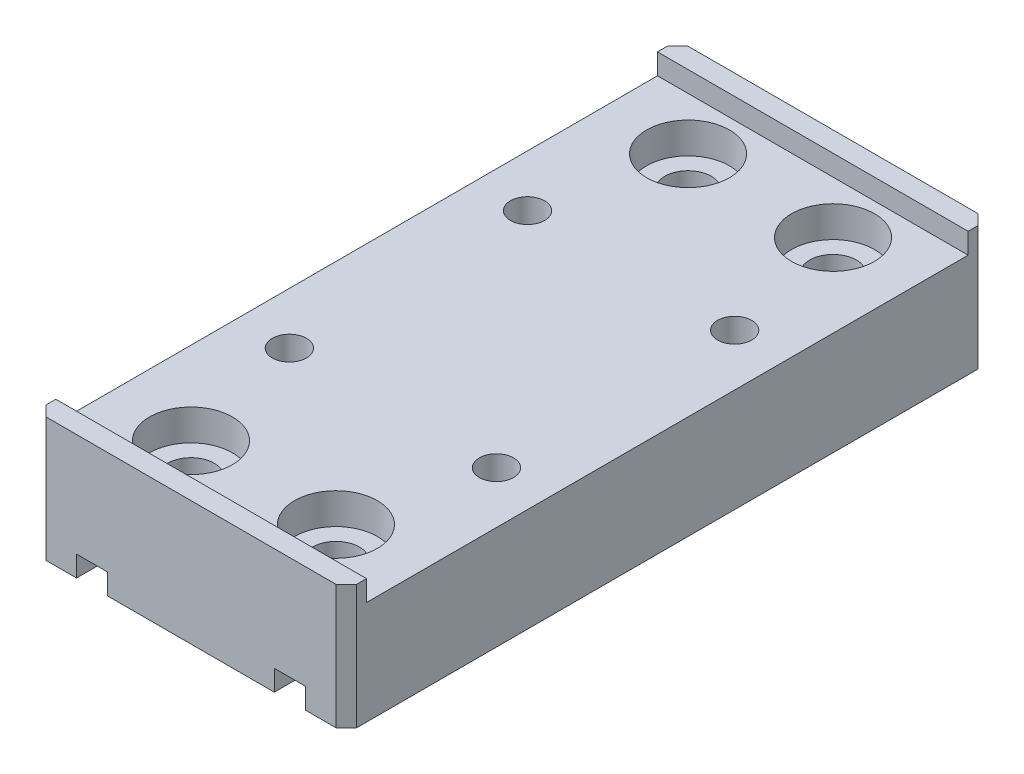
from build123d import *

# Parameters (mm, degrees)
SKETCH_1_W                = 30
SKETCH_1_H                = 62
EXTRUDE_1_DEPTH           = 12
SKETCH_2_W                = 22.1
SKETCH_2_H                = 56.1
CUT_EXTRUDE_1_DEPTH       = 2
SKETCH_3_W                = 3
SKETCH_3_H                = 72.139143417
CUT_EXTRUDE_2_DEPTH       = 2
SKETCH_4_W                = 86.092630608
SKETCH_4_H                = 58.1
CUT_EXTRUDE_3_DEPTH       = 2
HOLE_WIZARD_M4_1_D        = 3.3
HOLE_WIZARD_1_D           = 4.5
HOLE_WIZARD_1_CBORE_D     = 8
HOLE_WIZARD_1_CBORE_DEPTH = 5
CHAMFER_1_SIZE            = 1


with BuildPart() as part:
    # 草图1 → 凸台-拉伸1 (new body)
    with BuildSketch(Plane(origin=(0, 0, 0), x_dir=(1, 0, 0), z_dir=(0, 1, 0))):
        Rectangle(SKETCH_1_W, SKETCH_1_H)
    extrude(amount=EXTRUDE_1_DEPTH)

    # 草图2 → 切除-拉伸1 (cut)
    with BuildSketch(Plane.XZ):
        Rectangle(SKETCH_2_W, SKETCH_2_H)
    extrude(amount=-CUT_EXTRUDE_1_DEPTH, mode=Mode.SUBTRACT)

    # 草图3 → 切除-拉伸2 (cut)
    with BuildSketch(Plane.XZ):
        with Locations((-9.55, 0.756704302)):
            Rectangle(SKETCH_3_W, SKETCH_3_H)
    cut_extrude_2 = extrude(amount=-CUT_EXTRUDE_2_DEPTH, mode=Mode.SUBTRACT)

    # 镜向1: 切除-拉伸2 across plane
    add(cut_extrude_2.mirror(Plane(origin=(0, 0, 0), x_dir=(0, 0, 1), z_dir=(1, 0, 0))), mode=Mode.SUBTRACT)

    # 草图4 → 切除-拉伸3 (cut)
    with BuildSketch(Plane(origin=(0, 12, 0), x_dir=(1, 0, 0), z_dir=(0, 1, 0))):
        Rectangle(SKETCH_4_W, SKETCH_4_H)
    extrude(amount=-CUT_EXTRUDE_3_DEPTH, mode=Mode.SUBTRACT)

    # M4 螺纹孔1 (through all)
    with Locations(Plane(origin=(0, 10, 0), x_dir=(1, 0, 0), z_dir=(0, 1, 0))):
        with Locations((-10, 11.5), (10, 11.5), (-10, -11.5), (10, -11.5)):
            Hole(HOLE_WIZARD_M4_1_D / 2)

    # 打孔尺寸(%根据)开槽圆柱头螺钉的类型1 (through all)
    with Locations(Plane(origin=(0, 12, 0), x_dir=(1, 0, 0), z_dir=(0, 1, 0))):
        with Locations((-7, 24), (7, 24), (-7, -24), (7, -24)):
            CounterBoreHole(HOLE_WIZARD_1_D / 2, HOLE_WIZARD_1_CBORE_D / 2, HOLE_WIZARD_1_CBORE_DEPTH)

    # 倒角1
    chamfer_1_edges = [part.edges().sort_by_distance(p)[0] for p in [
        (15, 6, 31),
        (-15, 6, 31),
        (-15, 6, -31),
        (15, 6, -31),
    ]]
    chamfer(chamfer_1_edges, length=CHAMFER_1_SIZE)


solid = part.part
